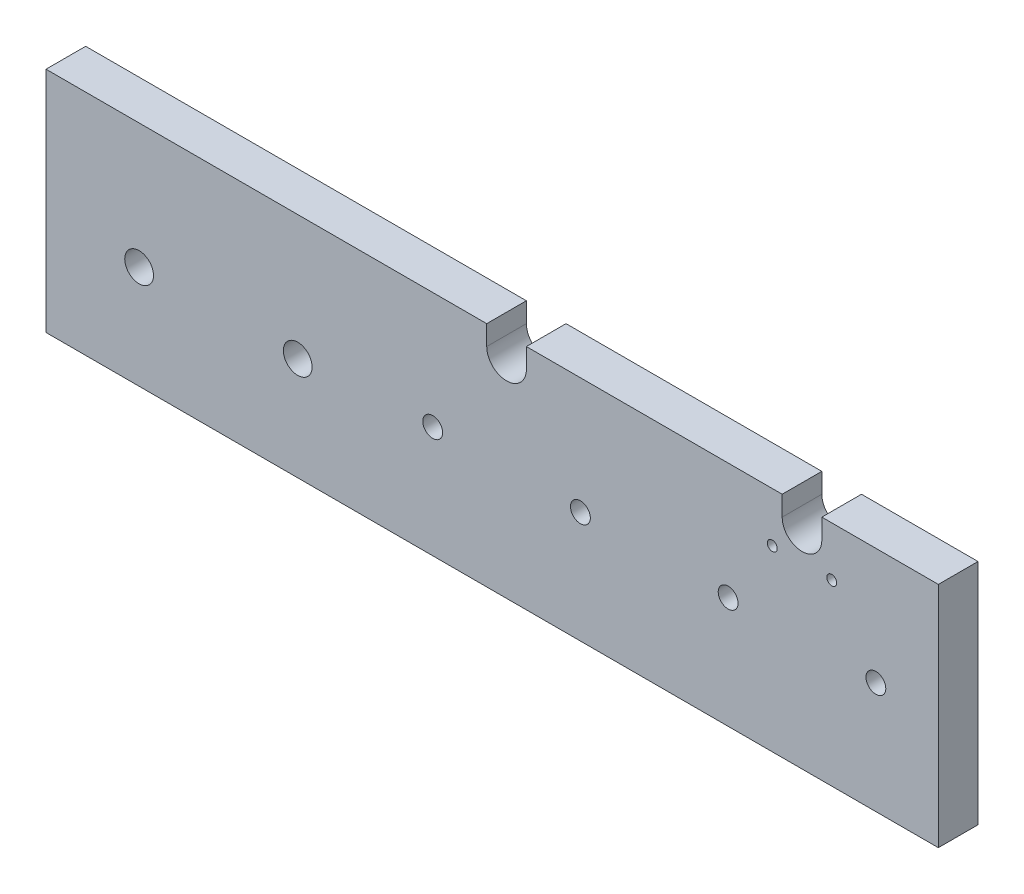
from build123d import *

# Parameters (mm, degrees)
SKETCH1_W           = 900
SKETCH1_H           = 230
BOSS_EXTRUDE1_DEPTH = 20
SKETCH2_R           = 10
CUT_EXTRUDE1_DEPTH  = 467.181295206
CUT_EXTRUDE2_DEPTH  = 467.181295206
LPATTERN1_COUNT     = 2
LPATTERN1_PITCH     = 298
LPATTERN2_COUNT     = 4
LPATTERN2_PITCH     = 149
SKETCH5_R           = 5
CUT_EXTRUDE4_DEPTH  = 467.181295206
SKETCH6_R           = 14.5
CUT_EXTRUDE5_DEPTH  = 467.181295206


with BuildPart() as part:
    # Sketch1 → Boss-Extrude1 (new, symmetric)
    with BuildSketch(Plane.XY):
        Rectangle(SKETCH1_W, SKETCH1_H)
    extrude(amount=BOSS_EXTRUDE1_DEPTH, both=True)

    # Sketch2 → Cut-Extrude1 (cut, through all)
    with BuildSketch(Plane.XY.offset(20)):
        with Locations((387, -2.5)):
            Circle(SKETCH2_R)
    cut_extrude1 = extrude(amount=-CUT_EXTRUDE1_DEPTH, mode=Mode.SUBTRACT)

    # Sketch3 → Cut-Extrude2 (cut, through all)
    with BuildSketch(Plane.XY.offset(20)):
        with BuildLine():
            Line((332.5, 115), (332.5, 95))
            ThreePointArc((332.5, 95), (312.5, 75), (292.5, 95))
            Line((292.5, 95), (292.5, 115))
            ThreePointArc((292.5, 115), (312.5, 135), (332.5, 115))
        make_face()
    cut_extrude2 = extrude(amount=-CUT_EXTRUDE2_DEPTH, mode=Mode.SUBTRACT)

    # LPattern1: Cut-Extrude2 ×2
    with Locations(*[(-i * LPATTERN1_PITCH, 0, 0) for i in range(1, LPATTERN1_COUNT)]):
        add(cut_extrude2, mode=Mode.SUBTRACT)

    # LPattern2: Cut-Extrude1 ×4
    with Locations(*[(-i * LPATTERN2_PITCH, 0, 0) for i in range(1, LPATTERN2_COUNT)]):
        add(cut_extrude1, mode=Mode.SUBTRACT)

    # Sketch5 → Cut-Extrude4 (cut, through all)
    with BuildSketch(Plane(origin=(0, 0, -20), x_dir=(-1, 0, 0), z_dir=(0, 0, -1))):
        with Locations((-342.5, 65)):
            Circle(SKETCH5_R)
        with Locations(Location((-282.5, 65, 0), (0, 0, 180))):
            Circle(SKETCH5_R)
    extrude(amount=-CUT_EXTRUDE4_DEPTH, mode=Mode.SUBTRACT)

    # Sketch6 → Cut-Extrude5 (cut, through all)
    with BuildSketch(Plane(origin=(0, 0, -20), x_dir=(-1, 0, 0), z_dir=(0, 0, -1))):
        with Locations((356.1, -11)):
            Circle(SKETCH6_R)
        with Locations((196.1, -11)):
            Circle(SKETCH6_R)
    extrude(amount=-CUT_EXTRUDE5_DEPTH, mode=Mode.SUBTRACT)


solid = part.part
